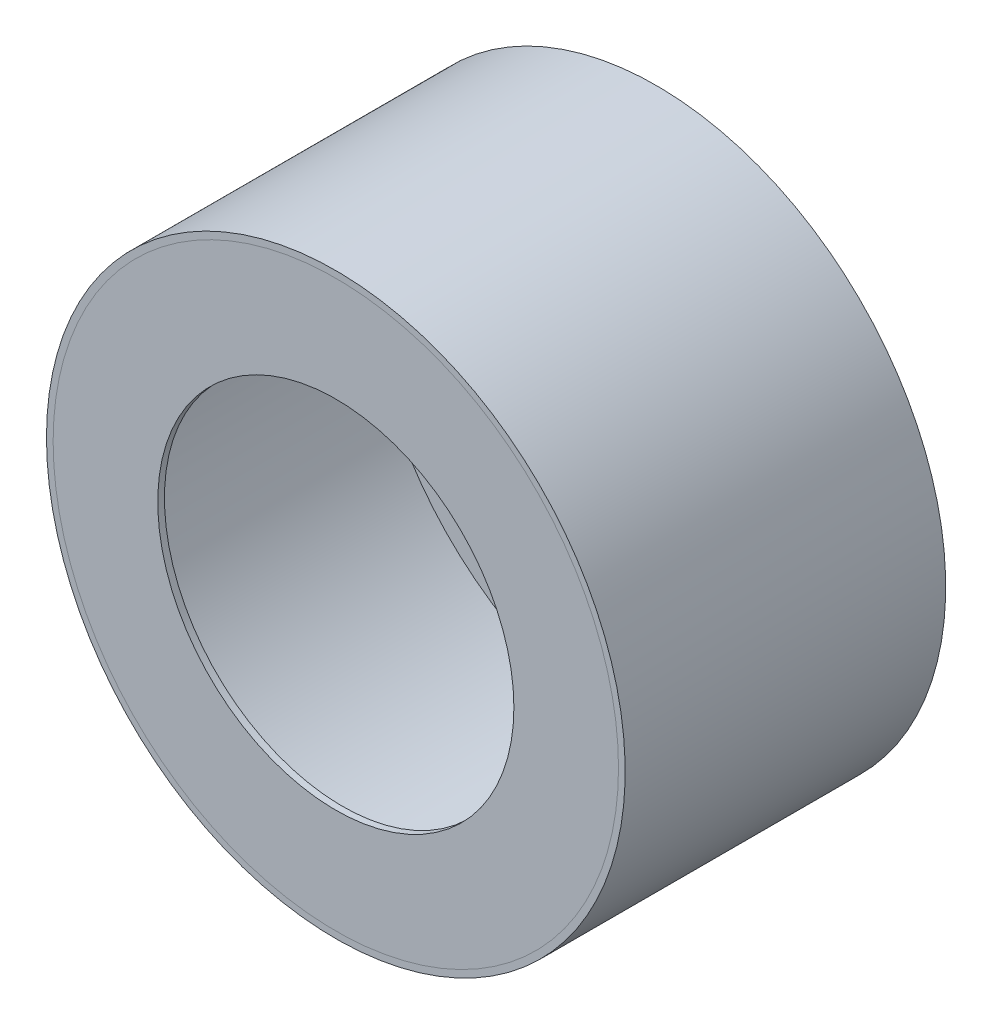
from build123d import *

# Parameters (mm, degrees)
SKETCH1_R           = 325
BOSS_EXTRUDE1_DEPTH = 360
SKETCH2_R           = 180
CUT_EXTRUDE1_DEPTH  = 584.823603497
CUT_EXTRUDE2_START  = -7.5
SKETCH3_R           = 317.5
CUT_EXTRUDE2_DEPTH  = 360
SKETCH4_R           = 5.5
SKETCH4_W           = 400
SKETCH4_H           = 200
CUT_EXTRUDE3_DEPTH  = 10
SKETCH5_R           = 317.5
SKETCH5_R_2         = 200
BOSS_EXTRUDE2_DEPTH = 7.5


with BuildPart() as part:
    # Sketch1 → Boss-Extrude1 (new body)
    with BuildSketch(Plane.XY):
        with Locations(Location((0, 0, 0), (0, 0, 180))):
            Circle(SKETCH1_R)
    extrude(amount=BOSS_EXTRUDE1_DEPTH)

    # Sketch2 → Cut-Extrude1 (cut, through all)
    with BuildSketch(Plane(origin=(0, 0, 0), x_dir=(-1, 0, 0), z_dir=(0, 0, -1))):
        Circle(SKETCH2_R)
    extrude(amount=-CUT_EXTRUDE1_DEPTH, mode=Mode.SUBTRACT)

    # Sketch3 → Cut-Extrude2 (cut)
    with BuildSketch(Plane(origin=(0, 0, 0), x_dir=(-1, 0, 0), z_dir=(0, 0, -1)).offset(CUT_EXTRUDE2_START)):
        Circle(SKETCH3_R)
    extrude(amount=-CUT_EXTRUDE2_DEPTH, mode=Mode.SUBTRACT)

    # Sketch4 → Cut-Extrude3 (cut)
    with BuildSketch(Plane(origin=(0, 0, 0), x_dir=(-1, 0, 0), z_dir=(0, 0, -1))):
        with Locations((-102.5, 177.535207776)):
            Circle(SKETCH4_R)
        with Locations((102.5, 177.535207776)):
            Circle(SKETCH4_R)
        with Locations((102.5, -177.535207776)):
            Circle(SKETCH4_R)
        with Locations((-102.5, -177.535207776)):
            Circle(SKETCH4_R)
        Rectangle(SKETCH4_W, SKETCH4_H)
    extrude(amount=-CUT_EXTRUDE3_DEPTH, mode=Mode.SUBTRACT)


with BuildPart() as body_2:
    # Sketch5 → Boss-Extrude2 (new body)
    with BuildSketch(Plane.XY.offset(360)):
        Circle(SKETCH5_R)
        Circle(SKETCH5_R_2, mode=Mode.SUBTRACT)
    extrude(amount=-BOSS_EXTRUDE2_DEPTH)


solid = Compound([part.part, body_2.part])
